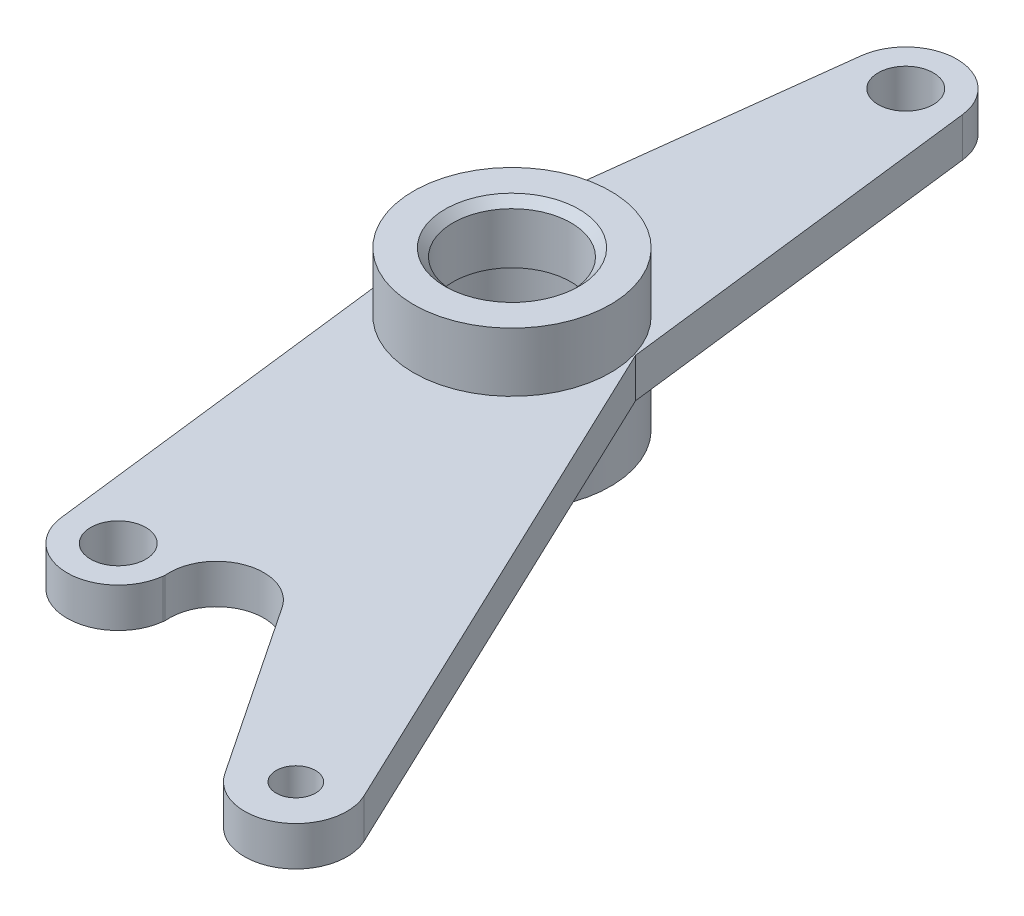
from build123d import *

# Parameters (mm, degrees)
SKETCH_1_R          = 25
SKETCH_1_R_2        = 15
EXTRUDE_1_DEPTH     = 20
SKETCH_2_R          = 15
SKETCH_2_R_2        = 7
SKETCH_2_R_3        = 5
EXTRUDE_2_DEPTH     = 5
CHAMFER_1_SIZE      = 2
SKETCH_3_R          = 17
CUT_EXTRUDE_1_DEPTH = 10


with BuildPart() as part:
    # 草图1 → 凸台-拉伸1 (new, symmetric)
    with BuildSketch(Plane(origin=(0, 0, 0), x_dir=(1, 0, 0), z_dir=(0, 1, 0))):
        with Locations(Location((0, 0, 0), (0, 0, 270))):
            Circle(SKETCH_1_R)
        with Locations(Location((0, 0, 0), (0, 0, 270))):
            Circle(SKETCH_1_R_2, mode=Mode.SUBTRACT)
    extrude(amount=EXTRUDE_1_DEPTH, both=True)

    # 草图2 → 凸台-拉伸2 (add, symmetric)
    with BuildSketch(Plane(origin=(0, 0, 0), x_dir=(1, 0, 0), z_dir=(0, 1, 0))):
        with BuildLine():
            Line((-12.906060592, 101.56), (-24.819347292, 3))
            ThreePointArc((-24.819347292, 3), (-25, 0), (-24.819347292, -3))
            Line((-24.819347292, -3), (-12.906060592, -101.56))
            ThreePointArc((-12.906060592, -101.56), (0, -113), (12.906060592, -101.56))
            Line((12.906060592, -101.56), (12.968643035, -101.042248202))
            ThreePointArc((12.968643035, -101.042248202), (20.91103038, -88.629202002), (34.896228635, -93.274572004))
            Line((34.896228635, -93.274572004), (64.19020383, -137.125189021))
            ThreePointArc((64.19020383, -137.125189021), (81.416898698, -141.209712173), (86.742245765, -124.325310375))
            Line((86.742245765, -124.325310375), (24.330246726, 7.046385599))
            Line((24.330246726, 7.046385599), (12.906060592, 101.56))
            ThreePointArc((12.906060592, 101.56), (0, 113), (-12.906060592, 101.56))
        make_face()
        with Locations(Location((0, 0, 0), (0, 0, 270))):
            Circle(SKETCH_2_R, mode=Mode.SUBTRACT)
        with Locations(Location((0, 100, 0), (0, 0, 270))):
            Circle(SKETCH_2_R_2, mode=Mode.SUBTRACT)
        with Locations(Location((0, -100, 0), (0, 0, 90))):
            Circle(SKETCH_2_R_2, mode=Mode.SUBTRACT)
        with Locations(Location((75, -129.903810568, 0), (0, 0, 270))):
            Circle(SKETCH_2_R_3, mode=Mode.SUBTRACT)
    extrude(amount=EXTRUDE_2_DEPTH, both=True)

    # 倒角1
    chamfer_1_edges = [part.edges().sort_by_distance(p)[0] for p in [
        (0, -20, -15),
        (0, 20, -15),
    ]]
    chamfer(chamfer_1_edges, length=CHAMFER_1_SIZE)

    # 草图3 → 切除-拉伸1 (cut)
    with BuildSketch(Plane(origin=(0, 5, 0), x_dir=(1, 0, 0), z_dir=(0, 1, 0))):
        with Locations(Location((0, 0, 0), (0, 0, 270))):
            Circle(SKETCH_3_R)
    extrude(amount=-CUT_EXTRUDE_1_DEPTH, mode=Mode.SUBTRACT)


solid = part.part
